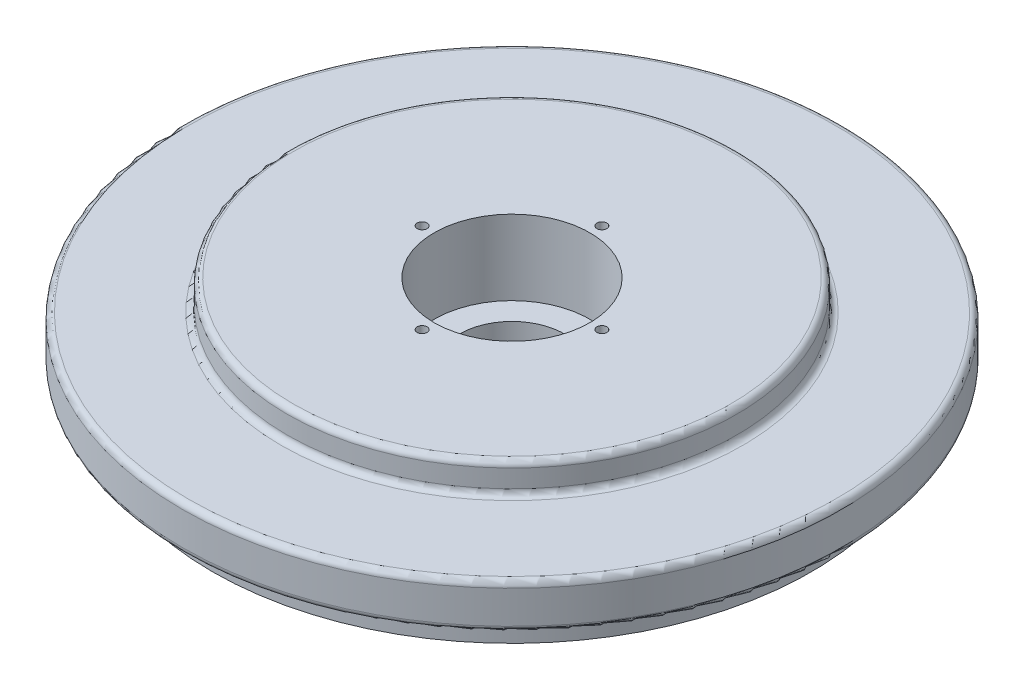
from build123d import *

# Parameters (mm, degrees)
SKETCH1_R           = 100
BOSS_EXTRUDE1_DEPTH = 10
SKETCH2_R           = 110
BOSS_EXTRUDE2_DEPTH = 15
SKETCH3_R           = 75
BOSS_EXTRUDE3_DEPTH = 10
FILLET1_R           = 2
SKETCH4_R           = 26
CUT_EXTRUDE1_DEPTH  = 25
SKETCH5_R           = 17.5
CUT_EXTRUDE2_DEPTH  = 158.559512566
CIRPATTERN1_COUNT   = 4
FILLET2_R           = 2


with BuildPart() as part:
    # Sketch1 → Boss-Extrude1 (new body)
    with BuildSketch(Plane(origin=(0, 0, 0), x_dir=(1, 0, 0), z_dir=(0, 1, 0))):
        with Locations(Location((0, 0, 0), (0, 0, 270))):
            Circle(SKETCH1_R)
    extrude(amount=BOSS_EXTRUDE1_DEPTH)

    # Sketch2 → Boss-Extrude2 (add)
    with BuildSketch(Plane(origin=(0, 10, 0), x_dir=(1, 0, 0), z_dir=(0, 1, 0))):
        with Locations(Location((0, 0, 0), (0, 0, 270))):
            Circle(SKETCH2_R)
    extrude(amount=BOSS_EXTRUDE2_DEPTH)

    # Sketch3 → Boss-Extrude3 (add)
    with BuildSketch(Plane(origin=(0, 25, 0), x_dir=(1, 0, 0), z_dir=(0, 1, 0))):
        with Locations(Location((0, 0, 0), (0, 0, 270))):
            Circle(SKETCH3_R)
    extrude(amount=BOSS_EXTRUDE3_DEPTH)

    # Fillet1
    fillet1_edges = [part.edges().sort_by_distance(p)[0] for p in [
        (0, 25, -75),
        (0, 35, -75),
    ]]
    fillet(fillet1_edges, radius=FILLET1_R)

    # Sketch4 → Cut-Extrude1 (cut)
    with BuildSketch(Plane(origin=(0, 35, 0), x_dir=(1, 0, 0), z_dir=(0, 1, 0))):
        with Locations(Location((0, 0, 0), (0, 0, 270))):
            Circle(SKETCH4_R)
    extrude(amount=-CUT_EXTRUDE1_DEPTH, mode=Mode.SUBTRACT)

    # Sketch5 → Cut-Extrude2 (cut, through all)
    with BuildSketch(Plane(origin=(0, 10, 0), x_dir=(1, 0, 0), z_dir=(0, 1, 0))):
        with Locations(Location((0, 0, 0), (0, 0, 270))):
            Circle(SKETCH5_R)
    extrude(amount=-CUT_EXTRUDE2_DEPTH, mode=Mode.SUBTRACT)

    # Sketch8 → M4 Tapped Hole1 (revolve, cut)
    with BuildSketch(Plane(origin=(0, 35, -30), x_dir=(0, 0, 1), z_dir=(1, 0, 0))):
        Polygon((0, 0), (0, 11.091420021), (1.65, 10.1), (1.65, 0), align=None)
    m4_tapped_hole1 = revolve(axis=Axis((0, 41.35, -30), (0, -1, 0)), mode=Mode.SUBTRACT)

    # CirPattern1: M4 Tapped Hole1 ×4 about axis
    cirpattern1_axis = Axis((0, 0, 0), (0, 1, 0))
    for i in range(1, CIRPATTERN1_COUNT):
        add(m4_tapped_hole1.rotate(cirpattern1_axis, i * 360 / CIRPATTERN1_COUNT), mode=Mode.SUBTRACT)

    # Fillet2
    fillet2_edges = [part.edges().sort_by_distance(p)[0] for p in [
        (0, 10, -110),
        (0, 25, -110),
    ]]
    fillet(fillet2_edges, radius=FILLET2_R)


solid = part.part
